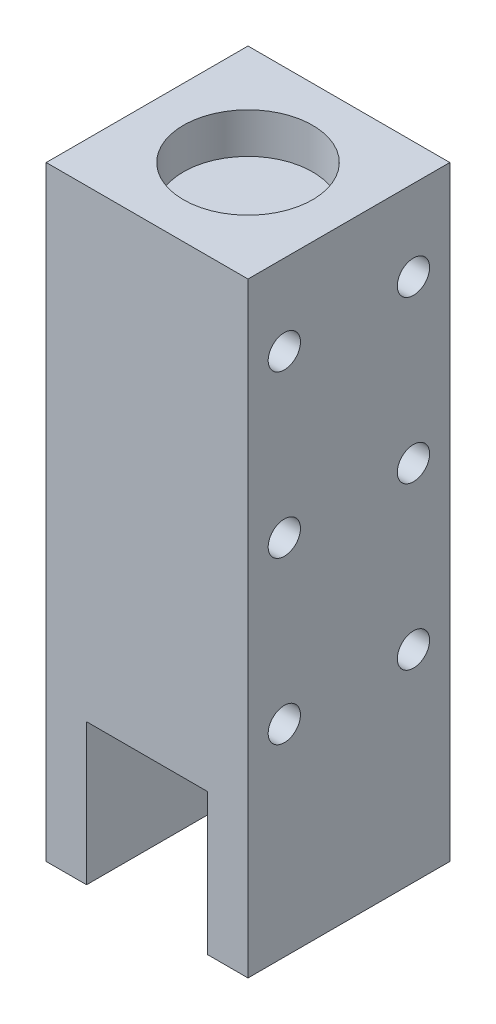
SolidWorks part; units mm, degrees
ref_plane "Front Plane" through (0, 0, 0) normal (0, 0, 1) x (1, 0, 0)
ref_plane "Top Plane" through (0, 0, 0) normal (0, 1, 0) x (1, 0, 0)
ref_plane "Right Plane" through (0, 0, 0) normal (1, 0, 0) x (0, 0, -1)
other "Configuration Table"
sketch "Sketch1" plane through (0, 0, 0) normal (0, 1, 0) x (1, 0, 0)
  line L1 (-25, 25) -> (25, 25)
  line L2 (-25, 25) -> (-25, -25)
  line L3 (-25, -25) -> (25, -25)
  line L4 (25, 25) -> (25, -25)
  line L5 (-25, 25) -> (25, -25) construction
  line L6 (-25, -25) -> (25, 25) construction
  point P0 (0, 0)
  dimension "D1" = 50
  dimension "D2" = 50
extrude "Boss-Extrude2" add sketch "Sketch1" along normal blind 150
sketch "Sketch2" plane through (0, 0, 0) normal (0, -1, 0) x (1, 0, 0)
  line L0 (25, -25) -> (-25, -25) construction
  line L1 (-15, 25) -> (15, 25)
  line L2 (-15, 25) -> (-15, -25)
  line L3 (-15, -25) -> (15, -25)
  line L4 (15, 25) -> (15, -25)
  line L5 (-15, 25) -> (15, -25) construction
  line L6 (-15, -25) -> (15, 25) construction
  point P0 (0, 0)
  dimension "D1" = 30
extrude "Cut-Extrude1" cut sketch "Sketch2" against normal blind 35
sketch "Sketch3" plane through (0, 150, 0) normal (0, 1, 0) x (1, 0, 0)
  line L1 (-21, 21) -> (21, 21)
  line L2 (-21, 21) -> (-21, -21)
  line L3 (-21, -21) -> (21, -21)
  line L4 (21, 21) -> (21, -21)
  line L5 (-21, 21) -> (21, -21) construction
  line L6 (-21, -21) -> (21, 21) construction
  point P0 (0, 0)
  dimension "D1" = 42
  dimension "D2" = 42
sketch "Sketch4" plane through (0, 150, 0) normal (0, 1, 0) x (1, 0, 0)
  circle A0 centre (0, 0) radius 16
  dimension "D1" = 32
extrude "Cut-Extrude2" cut sketch "Sketch4" against normal blind 10
sketch "Sketch5" plane through (25, 0, 0) normal (1, 0, 0) x (0, 0, -1)
  line L0 (0, 0) -> (0, 90)
  circle A0 centre (-16, 50) radius 4
  circle A1 centre (-16, 90) radius 4
  circle A2 centre (-16, 130) radius 4
  circle A3 centre (16, 50) radius 4
  circle A4 centre (16, 90) radius 4
  circle A5 centre (16, 130) radius 4
  dimension "D4" = 8
  dimension "D5" = 8
  dimension "D6" = 8
  dimension "D1" = 90
  dimension "D2" = 80
  dimension "D3" = 32
extrude "Cut-Extrude3" cut sketch "Sketch5" against normal blind 10 contours A2 | A5 | A1 | A0 | A3 | A4
mirror "Mirror1" about plane through (0, 0, 0) normal (1, 0, 0) of "Cut-Extrude3"
